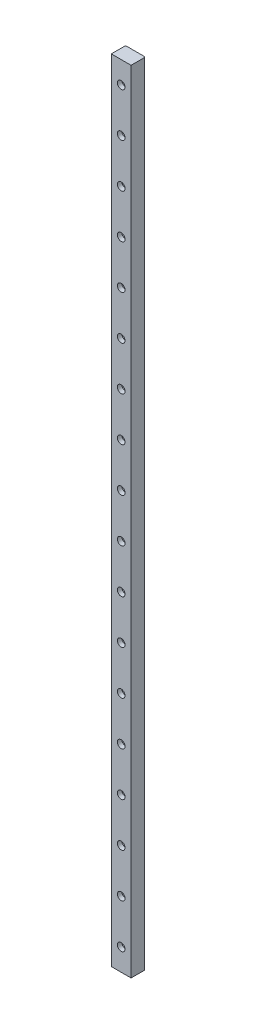
from build123d import *

# Parameters (mm, degrees)
SKETCH1_W           = 9
SKETCH1_H           = 6.5
BOSS_EXTRUDE1_DEPTH = 360
CHAMFER1_SIZE       = 0.3
SKETCH2_R           = 1.75
CUT_EXTRUDE1_DEPTH  = 37
LPATTERN1_COUNT     = 18
LPATTERN1_PITCH     = 20
SKETCH3_R           = 3
CUT_EXTRUDE2_DEPTH  = 4.5
LPATTERN2_COUNT     = 18
LPATTERN2_PITCH     = 20


with BuildPart() as part:
    # Sketch1 → Boss-Extrude1 (new body)
    with BuildSketch(Plane(origin=(0, 0, 0), x_dir=(1, 0, 0), z_dir=(0, 1, 0))):
        Rectangle(SKETCH1_W, SKETCH1_H)
    extrude(amount=BOSS_EXTRUDE1_DEPTH)

    # Chamfer1
    chamfer1_edges = [part.edges().sort_by_distance(p)[0] for p in [
        (-4.5, 180, -3.25),
        (4.5, 180, -3.25),
    ]]
    chamfer(chamfer1_edges, length=CHAMFER1_SIZE)

    # Sketch2 → Cut-Extrude1 (cut)
    with BuildSketch(Plane(origin=(0, 0, -3.25), x_dir=(-1, 0, 0), z_dir=(0, 0, -1))):
        with Locations((0, 10)):
            Circle(SKETCH2_R)
    cut_extrude1 = extrude(amount=-CUT_EXTRUDE1_DEPTH, mode=Mode.SUBTRACT)

    # LPattern1: Cut-Extrude1 ×18
    with Locations(*[(0, i * LPATTERN1_PITCH, 0) for i in range(1, LPATTERN1_COUNT)]):
        add(cut_extrude1, mode=Mode.SUBTRACT)

    # Sketch3 → Cut-Extrude2 (cut)
    with BuildSketch(Plane(origin=(0, 0, -3.25), x_dir=(-1, 0, 0), z_dir=(0, 0, -1))):
        with Locations((0, 10)):
            Circle(SKETCH3_R)
    cut_extrude2 = extrude(amount=-CUT_EXTRUDE2_DEPTH, mode=Mode.SUBTRACT)

    # LPattern2: Cut-Extrude2 ×18
    with Locations(*[(0, i * LPATTERN2_PITCH, 0) for i in range(1, LPATTERN2_COUNT)]):
        add(cut_extrude2, mode=Mode.SUBTRACT)


solid = part.part
